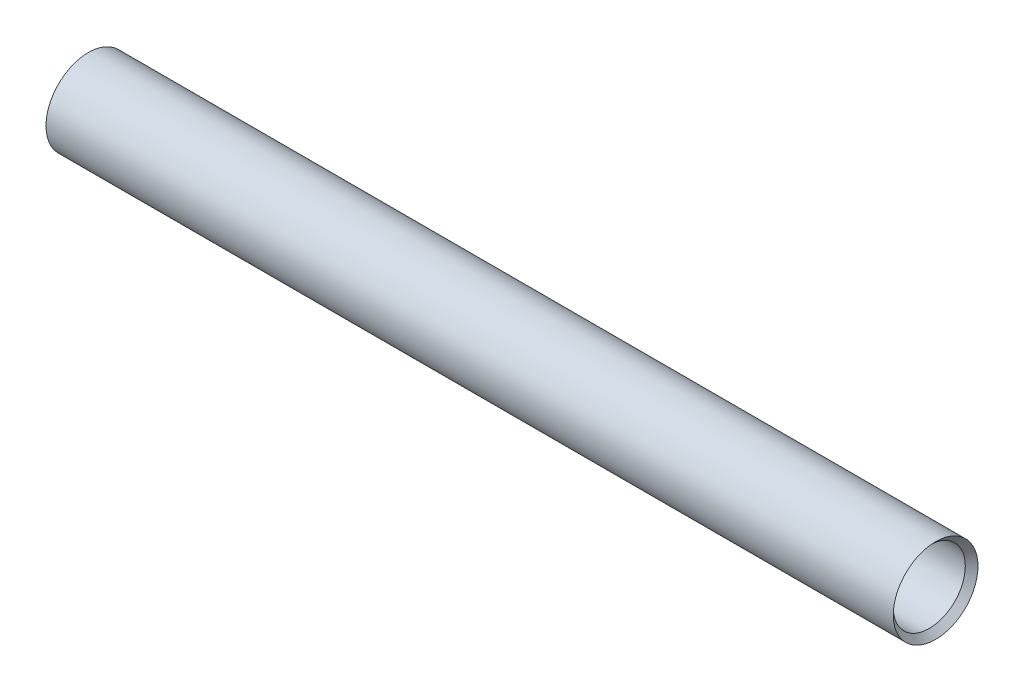
SolidWorks part; units mm, degrees
ref_plane "Front Plane" through (0, 0, 0) normal (0, 0, 1) x (1, 0, 0)
ref_plane "Top Plane" through (0, 0, 0) normal (0, 1, 0) x (1, 0, 0)
ref_plane "Right Plane" through (0, 0, 0) normal (1, 0, 0) x (0, 0, -1)
sketch "Sketch1" plane through (0, 0, 0) normal (0, 0, 1) x (1, 0, 0)
  line L0 (0, 0) -> (150.5518, 0) construction
  line L1 (0, 0) -> (0, 4)
  line L2 (0, 4) -> (80, 4)
  line L3 (80, 4) -> (80, 0)
  line L4 (0, 0) -> (80, 0)
  dimension "D1" = 4
  dimension "D2" = 80
revolve "Revolve1" add sketch "Sketch1" angle 360 about L0
hole_wizard "M8 Tapped Hole1" positions "3DSketch1" profile "Sketch2" tap size "M8" standard "GB"
sketch3d "3DSketch1"
  line L0 (80, 0, 0) -> (0, 0, 0) construction
  point P0 (80, 0, 0)
sketch "Sketch2" plane through (80, 0, 0) normal (0, 1, 0) x (0, 0, -1)
  line L0 (0, 0) -> (0, 20.7929)
  line L1 (0, 20.7929) -> (3.4, 18.75)
  line L2 (3.4, 18.75) -> (3.4, 0.625)
  line L3 (3.4, 0.625) -> (4.025, 0)
  line L5 (4.025, 0) -> (0, 0)
  line L6 (-3.4, 0.625) -> (-4.025, 0) construction
  line L10 (0, 20.7929) -> (-3.4, 18.75) construction
  line L11 (0, -6.35) -> (0, 107.95) construction
  dimension "螺纹孔钻头直径" = 6.8
  dimension "螺纹孔钻头深度" = 18.75
  dimension "近端锥形沉头孔直径" = 8.05
  dimension "近端锥形沉头孔角度" = 90
  dimension "导头角度" = 118
cosmetic thread "Cosmetic Thread1" parameters "D1"=15, "D2"=8
